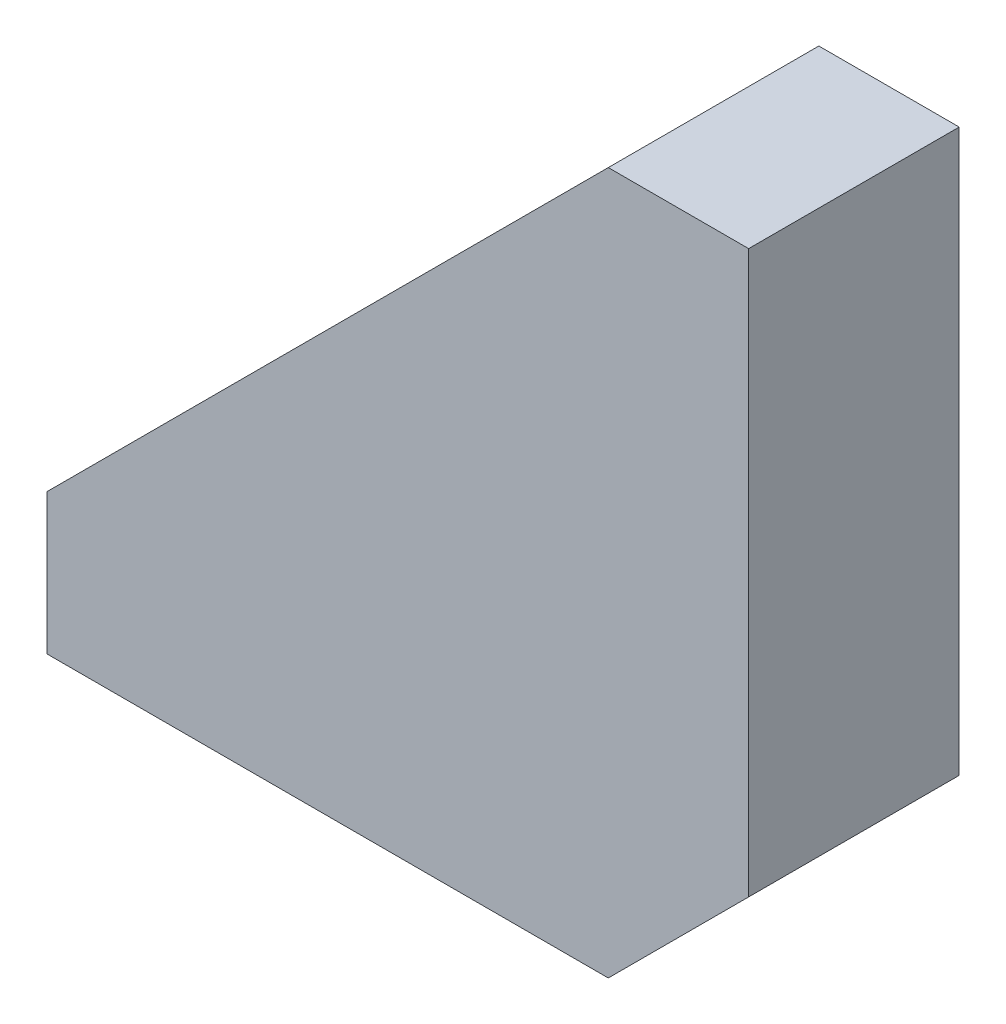
SolidWorks part; units mm, degrees
material "Q235B"
ref_plane "Front Plane" through (0, 0, 0) normal (0, 0, 1) x (1, 0, 0)
ref_plane "Top Plane" through (0, 0, 0) normal (0, 1, 0) x (1, 0, 0)
ref_plane "Right Plane" through (0, 0, 0) normal (1, 0, 0) x (0, 0, -1)
sketch "Sketch1" plane through (0, 0, 0) normal (0, 0, 1) x (1, 0, 0)
  line L0 (0, 0) -> (0, 10)
  line L1 (0, 10) -> (40, 50)
  line L2 (40, 50) -> (50, 50)
  line L3 (50, 50) -> (50, 10)
  line L4 (50, 10) -> (40, 0)
  line L5 (40, 0) -> (0, 0)
  dimension "D1" = 50
  dimension "D2" = 50
  dimension "D3" = 10
  dimension "D4" = 10
  dimension "D5" = 10
extrude "Boss-Extrude1" add sketch "Sketch1" along normal mid plane 15
